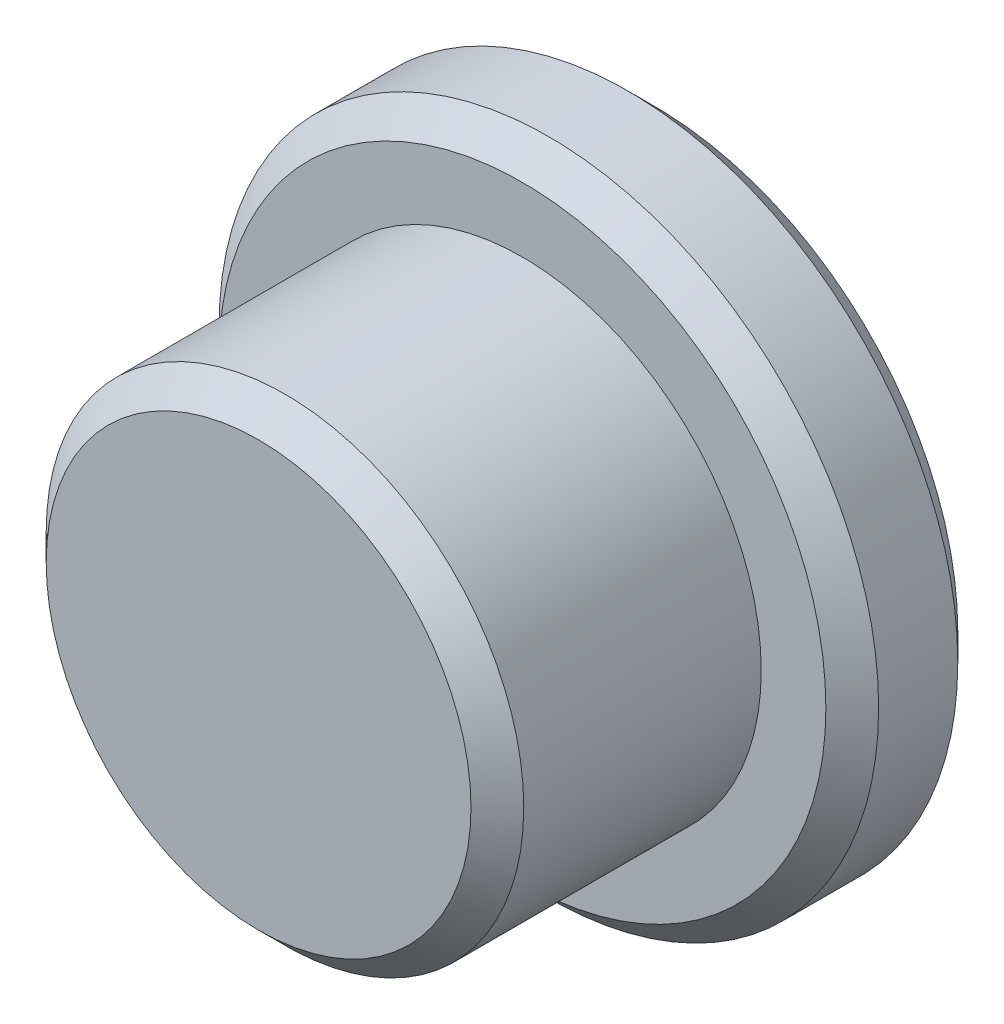
from build123d import *

# Parameters (mm, degrees)
CHAMFER1_SIZE = 1


with BuildPart() as part:
    # Sketch1 → Revolve1 (revolve)
    with BuildSketch(Plane(origin=(0, 0, 0), x_dir=(0, 0, -1), z_dir=(1, 0, 0)), mode=Mode.PRIVATE) as revolve1_sk:
        Polygon((15, 0), (15, 12.5), (10, 12.5), (10, 9.05), (0, 9.05), (0, 0), align=None)
    revolve(revolve1_sk.sketch.rotate(Axis((0, 0, 0), (0, 0, -1)), 90), axis=Axis((0, 0, 0), (0, 0, -1)))

    # Chamfer1
    chamfer1_edges = [part.edges().sort_by_distance(p)[0] for p in [
        (-9.05, 0, 0),
        (-12.5, 0, -10),
        (-12.5, 0, -15),
    ]]
    chamfer(chamfer1_edges, length=CHAMFER1_SIZE)


solid = part.part
